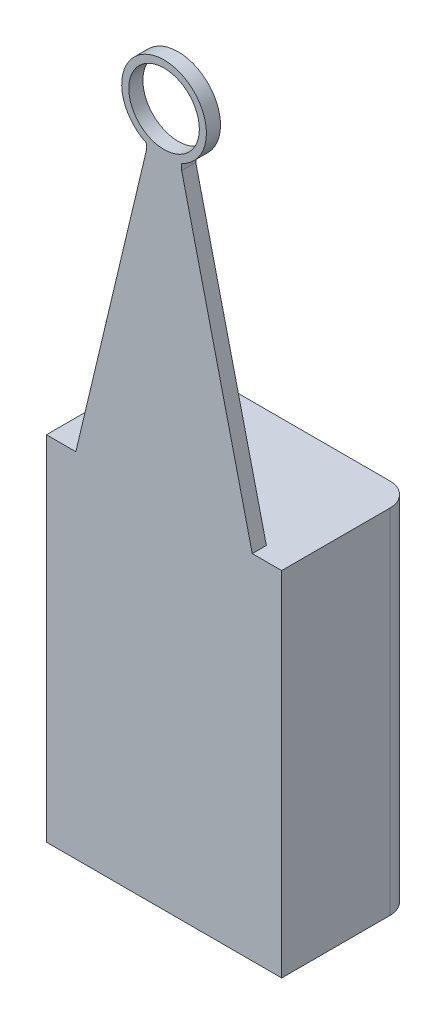
from build123d import *

# Parameters (mm, degrees)
SKETCH1_W           = 20
SKETCH1_H           = 11.2
BOSS_EXTRUDE1_DEPTH = 30
SKETCH2_R           = 3
BOSS_EXTRUDE2_DEPTH = 1.2
FILLET1_R           = 2
SKETCH3_R           = 0.6
BOSS_EXTRUDE3_DEPTH = 1


with BuildPart() as part:
    # Sketch1 → Boss-Extrude1 (new body)
    with BuildSketch(Plane(origin=(0, 0, 0), x_dir=(1, 0, 0), z_dir=(0, 1, 0))):
        Rectangle(SKETCH1_W, SKETCH1_H)
    extrude(amount=BOSS_EXTRUDE1_DEPTH)

    # Sketch2 → Boss-Extrude2 (add)
    with BuildSketch(Plane.XY.offset(5.6)):
        with BuildLine():
            Line((-1.5, 55.197386366), (-7.5, 30))
            Line((-7.5, 30), (7.5, 30))
            Line((7.5, 30), (1.5, 55.197386366))
            Line((1.5, 55.197386366), (1.5, 55.727386366))
            ThreePointArc((1.5, 55.727386366), (0, 62.6), (-1.5, 55.727386366))
            Line((-1.5, 55.727386366), (-1.5, 55.197386366))
        make_face()
        with Locations((0, 59)):
            Circle(SKETCH2_R, mode=Mode.SUBTRACT)
    extrude(amount=-BOSS_EXTRUDE2_DEPTH)

    # Fillet1
    fillet1_edges = [part.edges().sort_by_distance(p)[0] for p in [
        (-10, 15, -5.6),
        (10, 15, -5.6),
    ]]
    fillet(fillet1_edges, radius=FILLET1_R)

    # Sketch3 → Boss-Extrude3 (add)
    # profile 1 of 2: a face of its own
    with BuildSketch(Plane.XZ):
        with BuildLine():
            Line((6.5, -5.6), (4, -5.6))
            Line((4, -5.6), (4, -6.85))
            ThreePointArc((4, -6.85), (5.25, -8.1), (6.5, -6.85))
            Line((6.5, -6.85), (6.5, -5.6))
        make_face()
        with Locations(Location((5.25, -6.85, 0), (0, 0, 90))):
            Circle(SKETCH3_R, mode=Mode.SUBTRACT)
    # profile 2 of 2: a face of its own
    with BuildSketch(Plane.XZ):
        with BuildLine():
            Line((-6.5, -5.6), (-4, -5.6))
            Line((-4, -5.6), (-4, -6.85))
            ThreePointArc((-4, -6.85), (-5.25, -8.1), (-6.5, -6.85))
            Line((-6.5, -6.85), (-6.5, -5.6))
        make_face()
        with Locations(Location((-5.25, -6.85, 0), (0, 0, 270))):
            Circle(SKETCH3_R, mode=Mode.SUBTRACT)
    extrude(amount=-BOSS_EXTRUDE3_DEPTH)


solid = part.part
